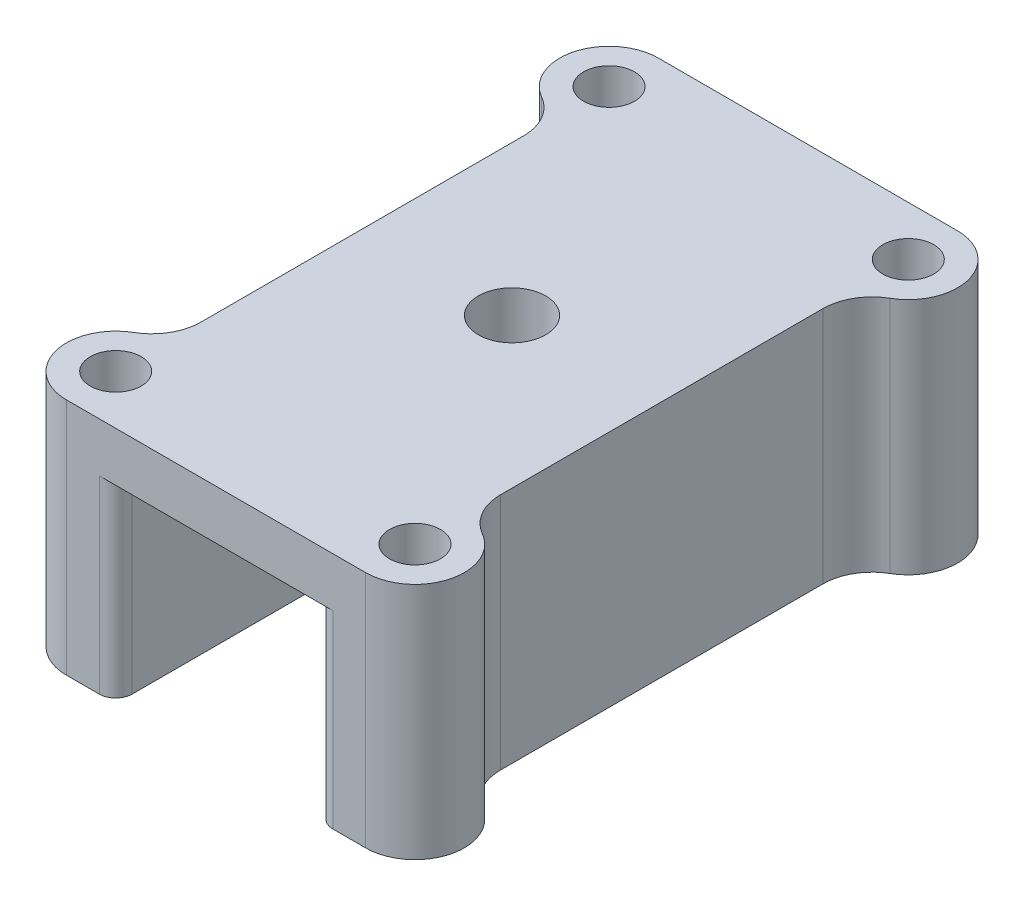
from build123d import *

# Parameters (mm, degrees)
EXTRUDE_1_DEPTH     = 36
SKETCH_2_R          = 3
EXTRUDE_2_DEPTH     = 14.5
SKETCH_3_R          = 1.55
SKETCH_3_R_2        = 2.05
CUT_EXTRUDE_1_DEPTH = 41.652921174
FILLET_1_R          = 3
FILLET_2_R          = 1


with BuildPart() as part:
    # 草图1 → 凸台-拉伸1 (new body)
    with BuildSketch(Plane.XY):
        Polygon((-6.1, 6), (6.1, 6), (6.1, -5.5), (9.1, -5.5), (9.1, 9), (-9.1, 9), (-9.1, -5.5), (-6.1, -5.5), align=None)
    extrude(amount=EXTRUDE_1_DEPTH)

    # 草图2 → 凸台-拉伸2 (add)
    with BuildSketch(Plane(origin=(0, 9, 0), x_dir=(1, 0, 0), z_dir=(0, 1, 0))):
        with Locations((9.1, -3)):
            Circle(SKETCH_2_R)
        with Locations((-9.1, -3)):
            Circle(SKETCH_2_R)
        with Locations((9.1, -33)):
            Circle(SKETCH_2_R)
        with Locations((-9.1, -33)):
            Circle(SKETCH_2_R)
    extrude(amount=-EXTRUDE_2_DEPTH)

    # 草图3 → 切除-拉伸1 (cut, through all)
    with BuildSketch(Plane(origin=(0, 9, 0), x_dir=(1, 0, 0), z_dir=(0, 1, 0))):
        with Locations(Location((9.1, -3, 0), (0, 0, 180))):
            Circle(SKETCH_3_R)
        with Locations(Location((-9.1, -33, 0), (0, 0, 180))):
            Circle(SKETCH_3_R)
        with Locations(Location((9.1, -33, 0), (0, 0, 180))):
            Circle(SKETCH_3_R)
        with Locations(Location((-9.1, -3, 0), (0, 0, 180))):
            Circle(SKETCH_3_R)
        with Locations(Location((0, -18, 0), (0, 0, 180))):
            Circle(SKETCH_3_R_2)
    extrude(amount=-CUT_EXTRUDE_1_DEPTH, mode=Mode.SUBTRACT)

    # 圆角1
    fillet_1_edges = [part.edges().sort_by_distance(p)[0] for p in [
        (9.1, 1.75, 6),
        (-9.1, 1.75, 6),
        (9.1, 1.75, 30),
        (-9.1, 1.75, 30),
    ]]
    fillet(fillet_1_edges, radius=FILLET_1_R)

    # 圆角2
    fillet_2_edges = [part.edges().sort_by_distance(p)[0] for p in [
        (6.1, 0.25, 0),
        (-6.1, 0.25, 0),
        (6.1, 0.25, 36),
        (-6.1, 0.25, 36),
    ]]
    fillet(fillet_2_edges, radius=FILLET_2_R)


solid = part.part
